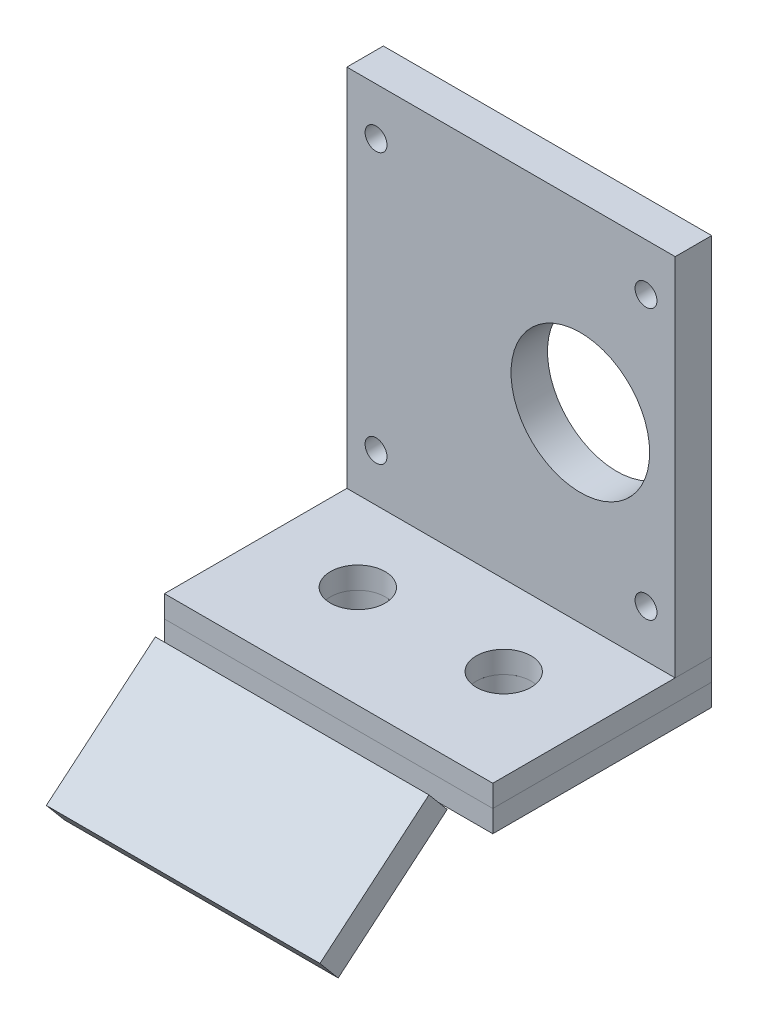
SolidWorks part; units mm, degrees
ref_plane "前视基准面" through (0, 0, 0) normal (0, 0, 1) x (1, 0, 0)
ref_plane "上视基准面" through (0, 0, 0) normal (0, 1, 0) x (1, 0, 0)
ref_plane "右视基准面" through (0, 0, 0) normal (1, 0, 0) x (0, 0, -1)
other "Configuration Table"
sketch "草图1" plane through (0, 0, 0) normal (0, 0, 1) x (1, 0, 0)
  line L0 (-45, -50) -> (45, -50)
  line L1 (-45, -50) -> (-45, 50)
  line L2 (-45, 50) -> (45, 50)
  line L3 (45, -50) -> (45, 50)
  line L4 (0, 50) -> (0, -50) construction
  line L5 (-45, 0) -> (45, 0) construction
  circle A0 centre (19, 0) radius 19
  circle A1 centre (-37, 37) radius 3
  circle A2 centre (37, 37) radius 3
  circle A3 centre (37, -37) radius 3
  circle A4 centre (-37, -37) radius 3
  point P0 (0, 0)
  dimension "D3" = 38
  dimension "D9" = 6
  dimension "D1" = 100
  dimension "D2" = 90
  dimension "D4" = 45
  dimension "D5" = 50
  dimension "D6" = 45
  dimension "D7" = 64
  dimension "D8" = 50
  dimension "D10" = 37
  dimension "D11" = 37
extrude "凸台-拉伸1" add sketch "草图1" along normal blind 10
sketch "草图2" plane through (0, -50, 0) normal (0, 1, 0) x (1, 0, 0)
  line L1 (-45, 0) -> (45, 0)
  line L2 (-45, 0) -> (-45, -60)
  line L3 (-45, -60) -> (45, -60)
  line L4 (45, 0) -> (45, -60)
  dimension "D1" = 60
  dimension "D2" = 90
extrude "凸台-拉伸2" add sketch "草图2" against normal blind 6 separate body
sketch "草图3" plane through (0, -56, 0) normal (0, -1, 0) x (-1, 0, 0)
  line L4 (45, -60) -> (45, 0)
  line L5 (-45, -60) -> (45, -60)
  line L6 (-45, 0) -> (-45, -60)
  line L7 (45, 0) -> (-45, 0)
  line L8 (45, -60) -> (45, 0)
  line L9 (-45, -60) -> (45, -60)
  line L10 (-45, 0) -> (-45, -60)
  line L11 (45, 0) -> (-45, 0)
  dimension "D1" = 0
extrude "凸台-拉伸3" add sketch "草图3" along normal blind 6 separate body
sketch "草图4" plane through (0, -62, 0) normal (0, -1, 0) x (-1, 0, 0)
  line L0 (0, 0) -> (0, -60.5669) construction
  line L1 (-45, 0) -> (45, 0) construction
  circle A0 centre (-20, -32) radius 7.5
  circle A1 centre (20, -32) radius 7.5
  dimension "D2" = 15
  dimension "D1" = 20
  dimension "D3" = 32
  dimension "D4" = 20
extrude "切除-拉伸1" cut sketch "草图4" against normal through all
sketch "草图5" plane through (-45, 0, 0) normal (1, 0, 0) x (0, 0, -1)
  line L0 (-62.5, -59.0206) -> (-57.5, -64.9794)
  line L5 (-60, -62) -> (0, -62) construction
  line L6 (-60, -62) -> (-60, -56) construction
  dimension "D1" = 50
  dimension "D2" = 5
  dimension "D3" = 2.5
extrude "拉伸-薄壁1" add sketch "草图5" along normal blind 75 separate body thin
sketch "草图6" plane through (0, -130.3168, 7.8971) normal (0, -0.6428, 0.766) x (-1, 0, 0)
  line L4 (-30, -81.9355) -> (-30, -89.7141)
  line L5 (45, -81.9355) -> (-30, -81.9355)
  line L6 (45, -89.7141) -> (45, -81.9355)
  line L7 (-30, -89.7141) -> (45, -89.7141)
  line L16 (-30, -81.9355) -> (-30, -89.7141)
  line L17 (45, -81.9355) -> (-30, -81.9355)
  line L18 (45, -89.7141) -> (45, -81.9355)
  line L19 (-30, -89.7141) -> (45, -89.7141)
  dimension "D1" = 0
extrude "凸台-拉伸4" add sketch "草图6" along normal blind 35
